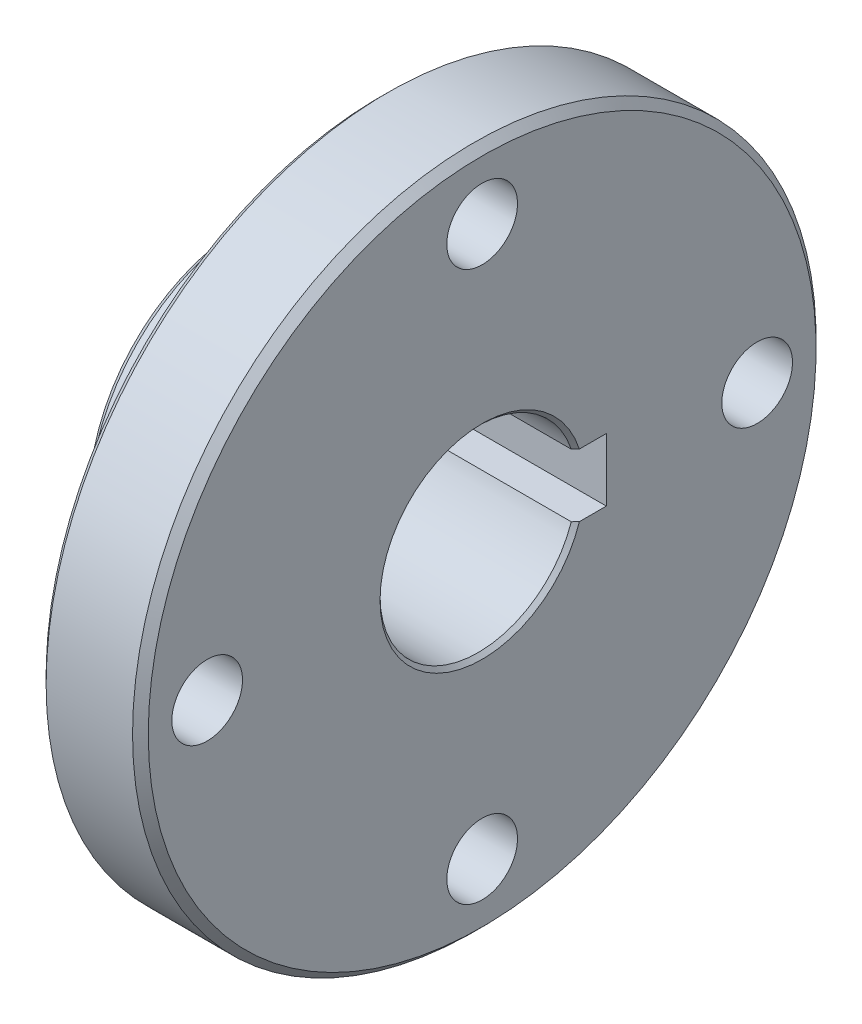
from build123d import *

# Parameters (mm, degrees)
CHAMFER1_SIZE      = 1
CHAMFER2_SIZE      = 0.5
FILLET1_R          = 5
CHAMFER3_SIZE      = 1
SKETCH2_R          = 4.5
CUT_EXTRUDE1_DEPTH = 20
SKETCH3_W          = 8.058064516
SKETCH3_H          = 8
CUT_EXTRUDE2_DEPTH = 69.443407279


with BuildPart() as part:
    # Sketch1 → Revolve1 (revolve)
    with BuildSketch(Plane.XY, mode=Mode.PRIVATE) as revolve1_sk:
        Polygon((0, 12.5), (0, 21), (17, 21), (17, 43.5), (30, 43.5), (30, 12.5), align=None)
    revolve(revolve1_sk.sketch.rotate(Axis((0, 0, 0), (1, 0, 0)), 90), axis=Axis((0, 0, 0), (1, 0, 0)))

    # Chamfer1
    chamfer1_edges = [part.edges().sort_by_distance(p)[0] for p in [
        (0, 0, -21),
    ]]
    chamfer(chamfer1_edges, length=CHAMFER1_SIZE)

    # Chamfer2
    chamfer2_edges = [part.edges().sort_by_distance(p)[0] for p in [
        (30, 0, -12.5),
        (0, 0, -12.5),
    ]]
    chamfer(chamfer2_edges, length=CHAMFER2_SIZE)

    # Fillet1
    fillet1_edges = [part.edges().sort_by_distance(p)[0] for p in [
        (17, 0, -21),
    ]]
    fillet(fillet1_edges, radius=FILLET1_R)

    # Chamfer3
    chamfer3_edges = [part.edges().sort_by_distance(p)[0] for p in [
        (17, 0, -43.5),
        (30, 0, -43.5),
    ]]
    chamfer(chamfer3_edges, length=CHAMFER3_SIZE)

    # Sketch2 → Cut-Extrude1 (cut)
    with BuildSketch(Plane.ZY.offset(-17)):
        with Locations((-35, 0)):
            Circle(SKETCH2_R)
        with Locations((0, -35)):
            Circle(SKETCH2_R)
        with Locations((0, 35)):
            Circle(SKETCH2_R)
        with Locations((35, 0)):
            Circle(SKETCH2_R)
    extrude(amount=-CUT_EXTRUDE1_DEPTH, mode=Mode.SUBTRACT)

    # Sketch3 → Cut-Extrude2 (cut, through all)
    with BuildSketch(Plane(origin=(30, 0, 0), x_dir=(0, 0, -1), z_dir=(1, 0, 0))):
        with Locations((11.770967742, 0)):
            Rectangle(SKETCH3_W, SKETCH3_H)
    extrude(amount=-CUT_EXTRUDE2_DEPTH, mode=Mode.SUBTRACT)


solid = part.part
